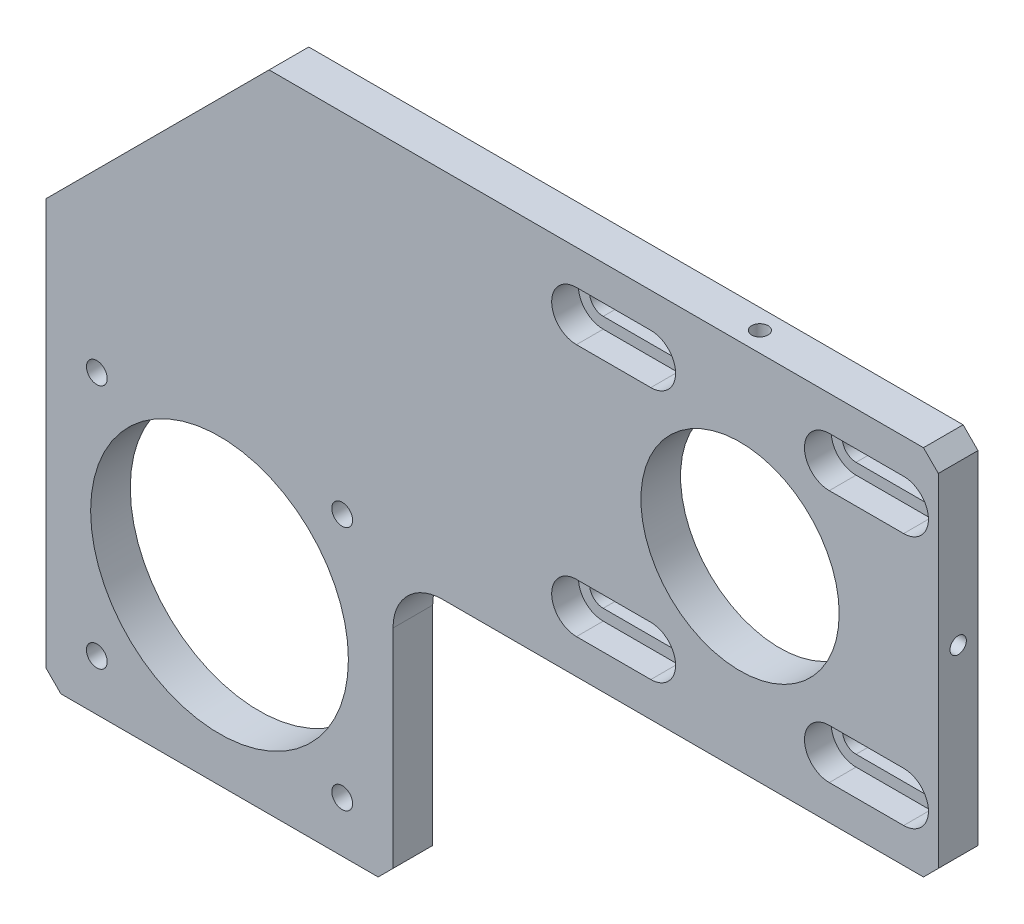
from build123d import *

# Parameters (mm, degrees)
SKETCH_2_W                     = 180
SKETCH_2_H                     = 130
EXTRUDE_1_DEPTH                = 4
SKETCH_3_W                     = 110
SKETCH_3_H                     = 55
CUT_EXTRUDE_1_DEPTH            = 8
SKETCH_4_R                     = 26
CUT_EXTRUDE_2_DEPTH            = 8
HOLE_WIZARD_M5_1_D             = 4.2
HOLE_WIZARD_M5_1_DEPTH         = 12.4
HOLE_WIZARD_M5_1_TIP           = 1.2618073
SKETCH_7_R                     = 20
CUT_EXTRUDE_3_DEPTH            = 8
HOLE_WIZARD_M4_1_D             = 3.3
HOLE_WIZARD_M4_1_DEPTH         = 12
HOLE_WIZARD_M4_1_TIP           = 0.991420021
HOLE_WIZARD_M4_2_D             = 3.3
HOLE_WIZARD_M4_2_DEPTH         = 12
HOLE_WIZARD_M4_2_TIP           = 0.991420021
CHAMFER_1_SIZE                 = 45
CHAMFER_2_SIZE                 = 3
FILLET_1_R                     = 10
HOLE_WIZARD_M5_1_2_D           = 5.5
HOLE_WIZARD_M5_1_2_DEPTH       = 10.1
HOLE_WIZARD_M5_1_2_CBORE_D     = 10
HOLE_WIZARD_M5_1_2_CBORE_DEPTH = 5.4
HOLE_WIZARD_M5_1_2_TIP         = 1.652366702
CUT_EXTRUDE_6_DEPTH            = 112.30588484
CUT_EXTRUDE_7_DEPTH            = 5.4
PATTERN_LINEAR_1_COUNT         = 2
PATTERN_LINEAR_1_PITCH         = 51
PATTERN_LINEAR_1_COUNT_DIR2    = 2
PATTERN_LINEAR_1_PITCH_DIR2    = 51
HOLE_WIZARD_M4_3_D             = 3.3
HOLE_WIZARD_M4_3_DEPTH         = 10.1
HOLE_WIZARD_M4_3_TIP           = 0.991420021
HOLE_WIZARD_M4_4_D             = 3.3
HOLE_WIZARD_M4_4_DEPTH         = 10.1
HOLE_WIZARD_M4_4_TIP           = 0.991420021


with BuildPart() as part:
    # 草图2 → 凸台-拉伸1 (new, symmetric)
    with BuildSketch(Plane.XY):
        Rectangle(SKETCH_2_W, SKETCH_2_H)
    extrude(amount=EXTRUDE_1_DEPTH, both=True)

    # 草图3 → 切除-拉伸1 (cut)
    with BuildSketch(Plane.XY.offset(4)):
        with Locations((35, -37.5)):
            Rectangle(SKETCH_3_W, SKETCH_3_H)
    extrude(amount=-CUT_EXTRUDE_1_DEPTH, mode=Mode.SUBTRACT)

    # 草图4 → 切除-拉伸2 (cut)
    with BuildSketch(Plane.XY.offset(4)):
        with Locations((-55, -30)):
            Circle(SKETCH_4_R)
    extrude(amount=-CUT_EXTRUDE_2_DEPTH, mode=Mode.SUBTRACT)

    # Hole Wizard M5 _1
    with Locations(Plane.XY.offset(4)):
        with Locations((-30.251262658, -54.748737342), (-79.748737342, -5.251262658), (-79.748737342, -54.748737342), (-30.251262658, -5.251262658)):
            Hole(HOLE_WIZARD_M5_1_D / 2, depth=HOLE_WIZARD_M5_1_DEPTH)
            with Locations((0, 0, -(HOLE_WIZARD_M5_1_DEPTH + HOLE_WIZARD_M5_1_TIP / 2))):  # 118° drill point
                Cone(0, HOLE_WIZARD_M5_1_D / 2, HOLE_WIZARD_M5_1_TIP, mode=Mode.SUBTRACT)

    # 草图7 → 切除-拉伸3 (cut)
    with BuildSketch(Plane.XY.offset(4)):
        with Locations((50, 27.5)):
            Circle(SKETCH_7_R)
    extrude(amount=-CUT_EXTRUDE_3_DEPTH, mode=Mode.SUBTRACT)

    # M4 螺纹孔1
    with Locations(Plane(origin=(0, 65, 0), x_dir=(1, 0, 0), z_dir=(0, 1, 0))):
        with Locations((50, 0)):
            Hole(HOLE_WIZARD_M4_1_D / 2, depth=HOLE_WIZARD_M4_1_DEPTH)
            with Locations((0, 0, -(HOLE_WIZARD_M4_1_DEPTH + HOLE_WIZARD_M4_1_TIP / 2))):  # 118° drill point
                Cone(0, HOLE_WIZARD_M4_1_D / 2, HOLE_WIZARD_M4_1_TIP, mode=Mode.SUBTRACT)

    # M4 螺纹孔2
    with Locations(Plane(origin=(0, -65, 0), x_dir=(-1, 0, 0), z_dir=(0, -1, 0))):
        with Locations((40, 0)):
            Hole(HOLE_WIZARD_M4_2_D / 2, depth=HOLE_WIZARD_M4_2_DEPTH)
            with Locations((0, 0, -(HOLE_WIZARD_M4_2_DEPTH + HOLE_WIZARD_M4_2_TIP / 2))):  # 118° drill point
                Cone(0, HOLE_WIZARD_M4_2_D / 2, HOLE_WIZARD_M4_2_TIP, mode=Mode.SUBTRACT)

    # 倒角1
    chamfer_1_edges = [part.edges().sort_by_distance(p)[0] for p in [
        (-90, 65, 0),
    ]]
    chamfer(chamfer_1_edges, length=CHAMFER_1_SIZE)

    # 倒角2
    chamfer_2_edges = [part.edges().sort_by_distance(p)[0] for p in [
        (90, -10, 0),
        (-20, -65, 0),
        (-90, -65, 0),
        (90, 65, 0),
    ]]
    chamfer(chamfer_2_edges, length=CHAMFER_2_SIZE)

    # 圆角1
    fillet_1_edges = [part.edges().sort_by_distance(p)[0] for p in [
        (-20, -10, 0),
    ]]
    fillet(fillet_1_edges, radius=FILLET_1_R)

    # Hole Wizard M5 _1 2
    with Locations(Plane.XY.offset(4)):
        with Locations((24.5, 53), (75.5, 53), (24.5, 2), (75.5, 2)):
            CounterBoreHole(HOLE_WIZARD_M5_1_2_D / 2, HOLE_WIZARD_M5_1_2_CBORE_D / 2, HOLE_WIZARD_M5_1_2_CBORE_DEPTH, depth=HOLE_WIZARD_M5_1_2_DEPTH)
            with Locations((0, 0, -(HOLE_WIZARD_M5_1_2_DEPTH + HOLE_WIZARD_M5_1_2_TIP / 2))):  # 118° drill point
                Cone(0, HOLE_WIZARD_M5_1_2_D / 2, HOLE_WIZARD_M5_1_2_TIP, mode=Mode.SUBTRACT)

    # 草图18 → 切除-拉伸6 (cut, through all)
    with BuildSketch(Plane.XY.offset(4)):
        with BuildLine():
            Line((17, 55.75), (32, 55.75))
            ThreePointArc((32, 55.75), (34.75, 53), (32, 50.25))
            Line((32, 50.25), (17, 50.25))
            ThreePointArc((17, 50.25), (14.25, 53), (17, 55.75))
        make_face()
    cut_extrude_6 = extrude(amount=-CUT_EXTRUDE_6_DEPTH, mode=Mode.SUBTRACT)

    # 草图19 → 切除-拉伸7 (cut)
    with BuildSketch(Plane.XY.offset(4)):
        with BuildLine():
            Line((17, 58), (32, 58))
            ThreePointArc((32, 58), (37, 53), (32, 48))
            Line((32, 48), (17, 48))
            ThreePointArc((17, 48), (12, 53), (17, 58))
        make_face()
    cut_extrude_7 = extrude(amount=-CUT_EXTRUDE_7_DEPTH, mode=Mode.SUBTRACT)

    # 阵列(线性)1: 切除-拉伸6, Cut-Extrude 7 2 × 2
    with Locations(*[(i * PATTERN_LINEAR_1_PITCH, -j * PATTERN_LINEAR_1_PITCH_DIR2, 0) for i in range(PATTERN_LINEAR_1_COUNT) for j in range(PATTERN_LINEAR_1_COUNT_DIR2) if (i, j) != (0, 0)]):
        add(cut_extrude_6, mode=Mode.SUBTRACT)
        add(cut_extrude_7, mode=Mode.SUBTRACT)

    # M4 螺纹孔3
    with Locations(Plane.ZY.offset(90)):
        with Locations((0, -15)):
            Hole(HOLE_WIZARD_M4_3_D / 2, depth=HOLE_WIZARD_M4_3_DEPTH)
            with Locations((0, 0, -(HOLE_WIZARD_M4_3_DEPTH + HOLE_WIZARD_M4_3_TIP / 2))):  # 118° drill point
                Cone(0, HOLE_WIZARD_M4_3_D / 2, HOLE_WIZARD_M4_3_TIP, mode=Mode.SUBTRACT)

    # M4 螺纹孔4
    with Locations(Plane(origin=(90, 0, 0), x_dir=(0, 0, -1), z_dir=(1, 0, 0))):
        with Locations((0, 30)):
            Hole(HOLE_WIZARD_M4_4_D / 2, depth=HOLE_WIZARD_M4_4_DEPTH)
            with Locations((0, 0, -(HOLE_WIZARD_M4_4_DEPTH + HOLE_WIZARD_M4_4_TIP / 2))):  # 118° drill point
                Cone(0, HOLE_WIZARD_M4_4_D / 2, HOLE_WIZARD_M4_4_TIP, mode=Mode.SUBTRACT)


solid = part.part
